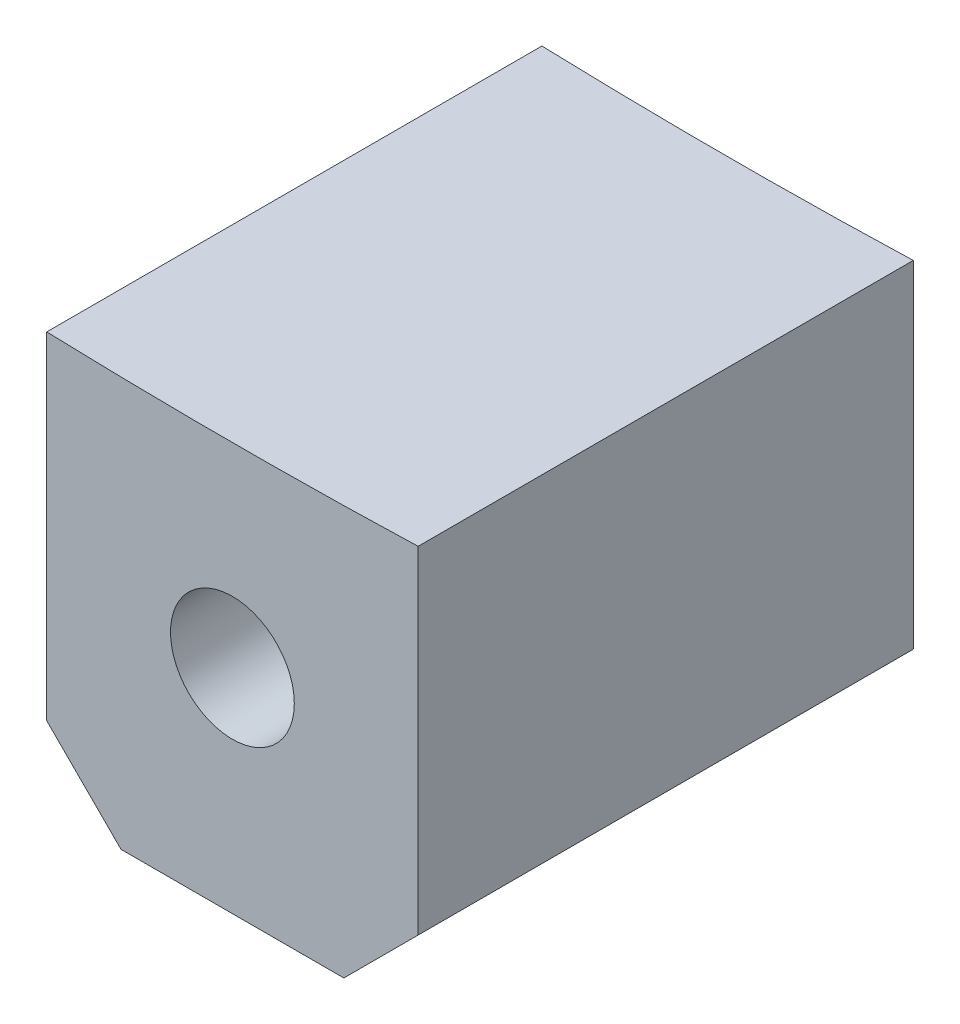
SolidWorks part; units mm, degrees
ref_plane "Front Plane" through (0, 0, 0) normal (0, 0, 1) x (1, 0, 0)
ref_plane "Top Plane" through (0, 0, 0) normal (0, 1, 0) x (1, 0, 0)
ref_plane "Right Plane" through (0, 0, 0) normal (1, 0, 0) x (0, 0, -1)
sketch "Sketch1" plane through (0, 0, 0) normal (0, 0, 1) x (1, 0, 0)
  line L0 (0, 0) -> (0, -325.9957) construction
  line L1 (-7.5, -231.1784) -> (-7.5, -247.7784)
  line L2 (-7.5, -247.7784) -> (7.5, -247.7784)
  line L3 (7.5, -247.7784) -> (7.5, -231.1784)
  arc A0 (-7.5, -231.1784) -> (7.5, -231.1784) centre (0, 0) ccw
  dimension "D1" = 462.6
  dimension "D2" = 15
  dimension "D3" = 16.6
extrude "Boss-Extrude1" add sketch "Sketch1" along normal blind 20
chamfer "Chamfer1" distance 3 angle 45 2 edges at (7.5, -247.7784, 10) (-7.5, -247.7784, 10)
sketch "Sketch2" plane through (0, 0, 20) normal (0, 0, 1) x (1, 0, 0)
  line L0 (0, -247.7784) -> (0, -229.1841) construction
  line L1 (-4.5, -247.7784) -> (4.5, -247.7784) construction
  point P0 (0, -239.1784)
  dimension "D1" = 8
hole_wizard "M6 Tapped Hole1" positions "Sketch5" profile "Sketch6" tap size "M6" standard "GB" end condition through all
sketch "Sketch5" plane through (0, 0, 20) normal (0, 0, 1) x (1, 0, 0)
  point P0 (0, -239.1784)
cosmetic thread "Cosmetic thread 1" parameters "D2"=6
sketch "Sketch6" plane through (0, -239.1784, 20) normal (1, 0, 0) x (0, -1, 0)
  line L0 (0, 0) -> (0, 20)
  line L1 (0, 20) -> (2.5, 20)
  line L2 (2.5, 20) -> (2.5, 0)
  line L5 (2.5, 0) -> (0, 0)
  line L11 (0, -6.35) -> (0, 107.95) construction
  dimension "通孔螺纹孔钻头直径" = 5
  dimension "通孔螺纹孔钻头深度" = 20
